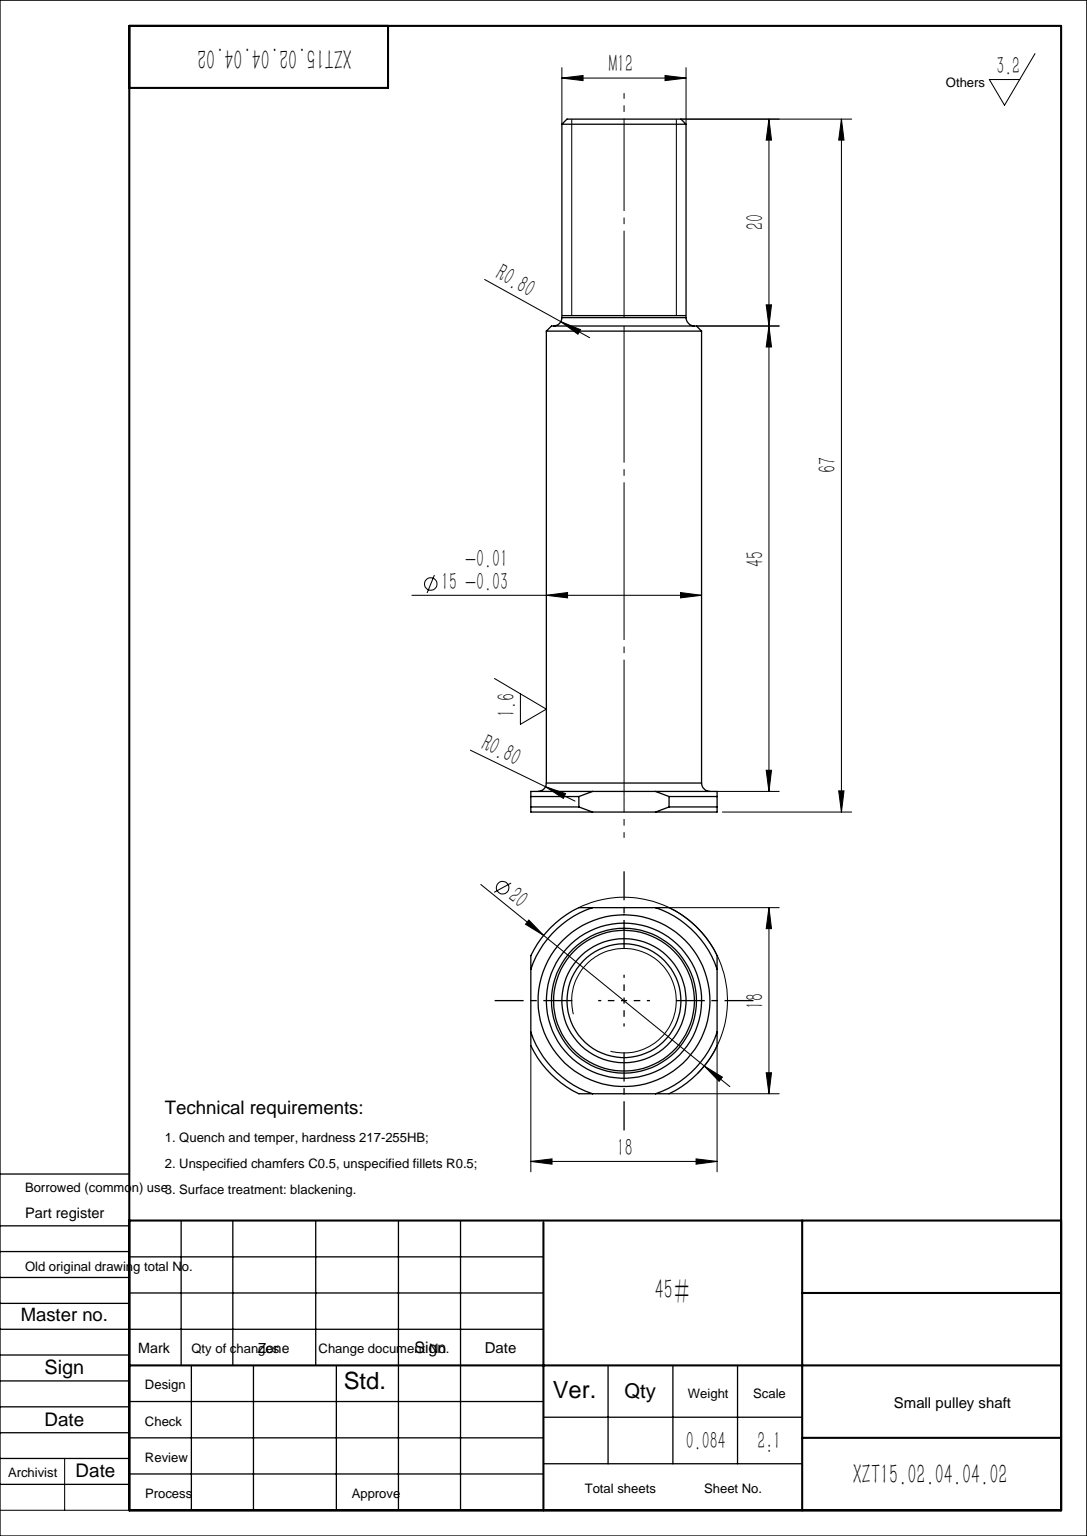
SolidWorks part; units mm, degrees
material "45#"
ref_plane "Front Plane" through (0, 0, 0) normal (0, 0, 1) x (1, 0, 0)
ref_plane "Top Plane" through (0, 0, 0) normal (0, 1, 0) x (1, 0, 0)
ref_plane "Right Plane" through (0, 0, 0) normal (1, 0, 0) x (0, 0, -1)
sketch "Sketch1" plane through (0, 0, 0) normal (0, 0, 1) x (1, 0, 0)
  line L0 (0, 0) -> (10, 0)
  line L1 (10, 0) -> (10, 2)
  line L2 (10, 2) -> (7.5, 2)
  line L3 (7.5, 2) -> (7.5, 47)
  line L4 (7.5, 47) -> (6, 47)
  line L5 (6, 47) -> (6, 67)
  line L6 (6, 67) -> (0, 67)
  line L7 (0, 67) -> (0, 0)
  line L8 (0, 0) -> (0, -4.6727) construction
  dimension "D1" = 20
  dimension "D2" = 15
  dimension "D3" = 12
  dimension "D4" = 20
  dimension "D5" = 65
  dimension "D6" = 67
revolve "Revolve1" add sketch "Sketch1" angle 360 about L8
cosmetic thread "Cosmetic Thread1" parameters "D1"=19, "D2"=10.106
chamfer "Chamfer1" distance 0.5 angle 45 4 edges at (0, 67, 6) (0, 0, 10) (0, 47, 7.5) (0, 2, 10)
fillet "Fillet1" radius 0.8 2 edges at (0, 47, 6) (0, 2, 7.5)
sketch "Sketch2" plane through (0, 0, 0) normal (0, 1, 0) x (1, 0, 0)
  line L1 (9, -9) -> (-9, -9)
  line L2 (9, -9) -> (9, 9)
  line L3 (9, 9) -> (-9, 9)
  line L4 (-9, -9) -> (-9, 9)
  line L5 (9, -9) -> (-9, 9) construction
  line L6 (9, 9) -> (-9, -9) construction
  point P0 (0, 0)
  dimension "D1" = 18
extrude "Cut-Extrude1" cut sketch "Sketch2" along normal blind 10 flip side to cut
